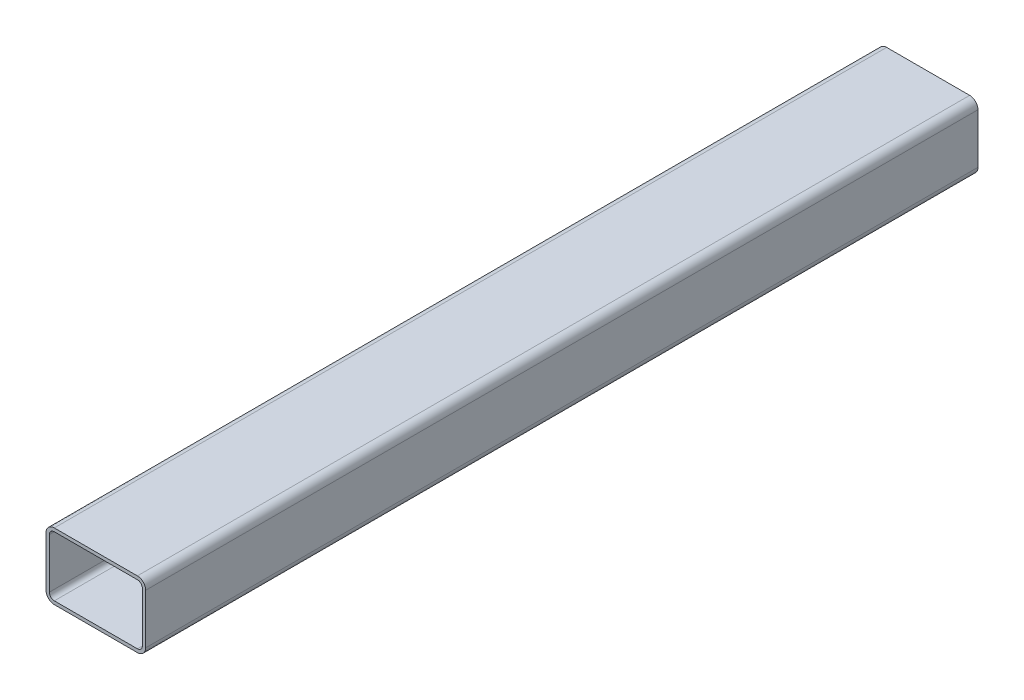
from build123d import *

# Parameters (mm, degrees)
SKETCH1_W           = 120
SKETCH1_H           = 80
BOSS_EXTRUDE1_DEPTH = 1002
FILLET1_R           = 10
SHELL1_T            = -4


with BuildPart() as part:
    # Sketch1 → Boss-Extrude1 (new body)
    with BuildSketch(Plane.XY):
        Rectangle(SKETCH1_W, SKETCH1_H)
    extrude(amount=BOSS_EXTRUDE1_DEPTH)

    # Fillet1
    fillet1_edges = [part.edges().sort_by_distance(p)[0] for p in [
        (-60, 40, 501),
        (60, 40, 501),
        (60, -40, 501),
        (-60, -40, 501),
    ]]
    fillet(fillet1_edges, radius=FILLET1_R)

    # Shell1
    shell1_openings = [part.faces().sort_by_distance(p)[0] for p in [
        (0, 0, 1002),
        (0, 0, 0),
    ]]
    offset(amount=SHELL1_T, openings=shell1_openings, kind=Kind.INTERSECTION)


solid = part.part
